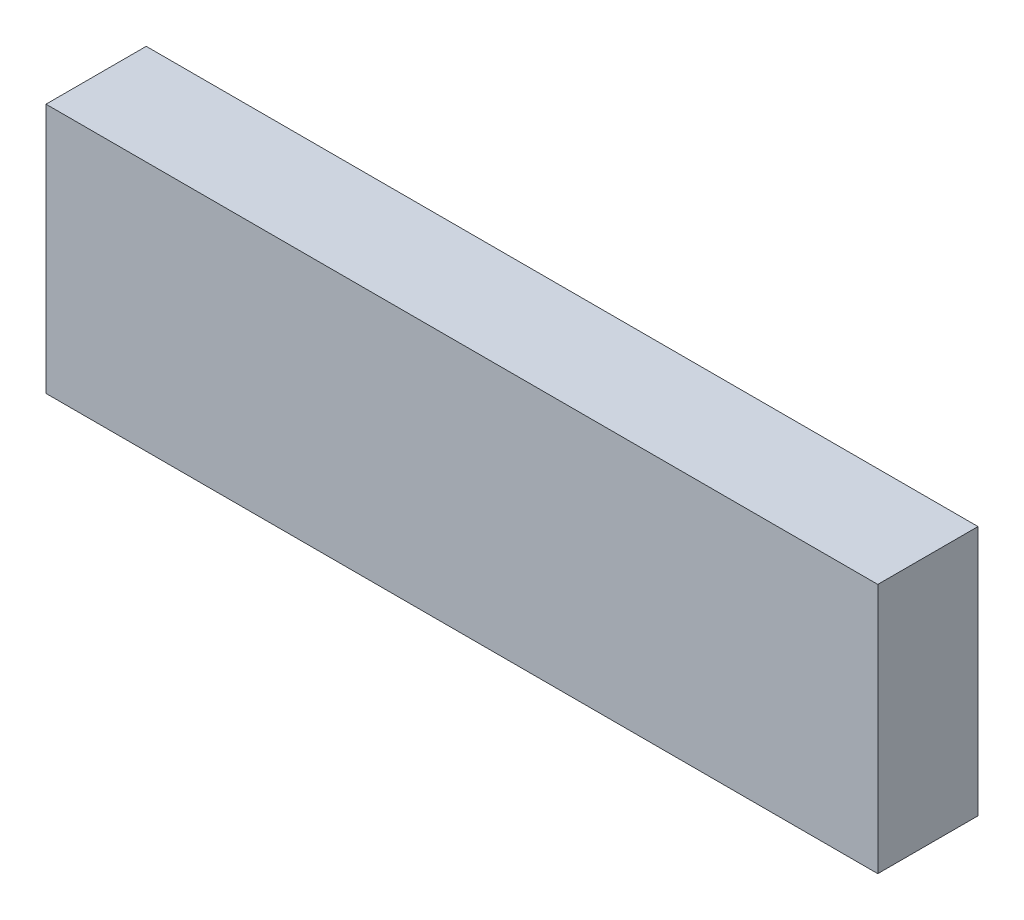
SolidWorks part; units mm, degrees
material "Q235B"
ref_plane "Front Plane" through (0, 0, 0) normal (0, 0, 1) x (1, 0, 0)
ref_plane "Top Plane" through (0, 0, 0) normal (0, 1, 0) x (1, 0, 0)
ref_plane "Right Plane" through (0, 0, 0) normal (1, 0, 0) x (0, 0, -1)
sketch "Sketch1" plane through (0, 0, 0) normal (0, 0, 1) x (1, 0, 0)
  line L1 (0, 0) -> (166, 0)
  line L2 (0, 0) -> (0, 50)
  line L3 (0, 50) -> (166, 50)
  line L4 (166, 0) -> (166, 50)
  dimension "D1" = 50
  dimension "D2" = 166
extrude "Boss-Extrude1" add sketch "Sketch1" along normal blind 20
